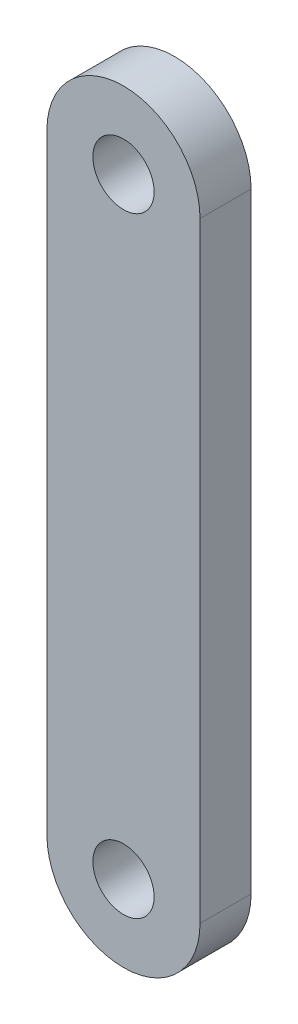
SolidWorks part; units mm, degrees
ref_plane "Front Plane" through (0, 0, 0) normal (0, 0, 1) x (1, 0, 0)
ref_plane "Top Plane" through (0, 0, 0) normal (0, 1, 0) x (1, 0, 0)
ref_plane "Right Plane" through (0, 0, 0) normal (1, 0, 0) x (0, 0, -1)
other "Configuration Table"
sketch "Sketch2" plane through (0, 0, -10) normal (0, 0, 1) x (1, 0, 0)
  line L0 (70, 40) -> (70, -79.6043)
  line L2 (100, -79.6043) -> (100, 40)
  arc A0 (100, 40) -> (70, 40) centre (85, 40) ccw
  circle A1 centre (85, 40) radius 6
  arc A2 (70, -79.6043) -> (100, -79.6043) centre (85, -79.6043) ccw
  circle A3 centre (85, -79.6043) radius 6
extrude "Boss-Extrude1" add sketch "Sketch2" along normal blind 10
